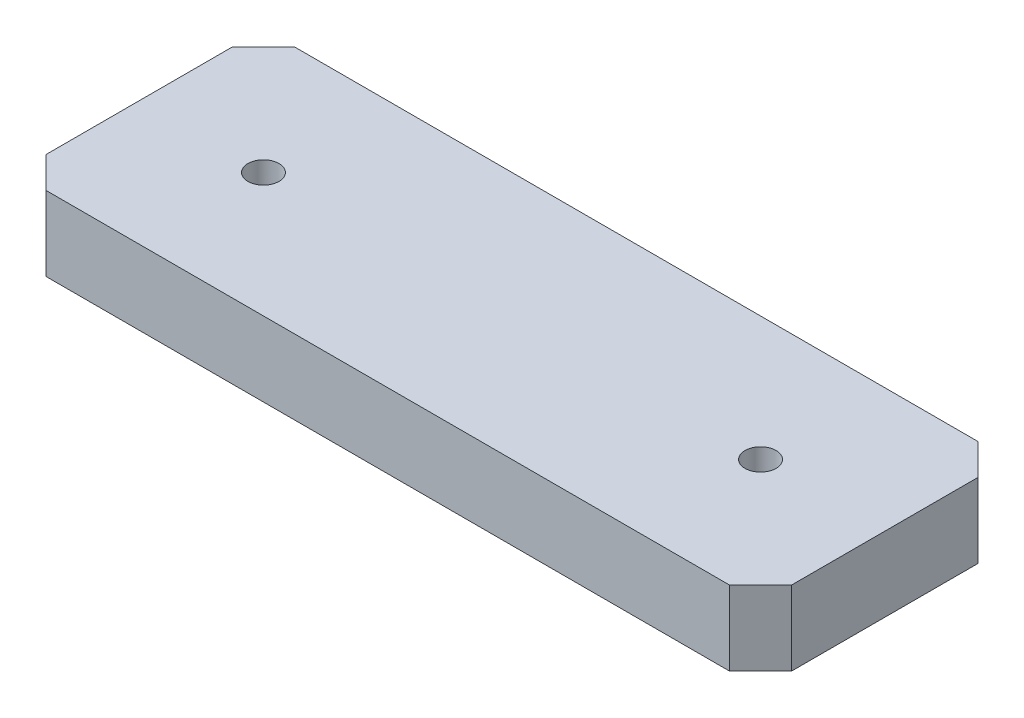
SolidWorks part; units mm, degrees
material "45#"
ref_plane "Front Plane" through (0, 0, 0) normal (0, 0, 1) x (1, 0, 0)
ref_plane "Top Plane" through (0, 0, 0) normal (0, 1, 0) x (1, 0, 0)
ref_plane "Right Plane" through (0, 0, 0) normal (1, 0, 0) x (0, 0, -1)
sketch "Sketch1" plane through (0, 0, 0) normal (0, 1, 0) x (1, 0, 0)
  line L0 (60, 20) -> (-60, -20) construction
  line L1 (-60, 20) -> (60, 20)
  line L2 (-60, 20) -> (-60, -20)
  line L3 (-60, -20) -> (60, -20)
  line L4 (60, 20) -> (60, -20)
  dimension "D1" = 120
  dimension "D2" = 40
extrude "Extrude1" add sketch "Sketch1" along normal mid plane 12
hole_wizard "M6 Tapped Hole1" positions "Sketch3" profile "Sketch2" tap size "M6" standard "ISO"
sketch "Sketch3" plane through (0, 6, 0) normal (0, 1, 0) x (-1, 0, 0)
  line L0 (-40, 0) -> (40, 0) construction
  line L2 (-60, 20) -> (-60, -20) construction
  point P0 (40, 0)
  point P1 (-40, 0)
  dimension "D1" = 20
sketch "Sketch2" plane through (-40, 6, 0) normal (1, 0, 0) x (0, 0, 1)
  line L0 (0, 0) -> (0, 16.5022)
  line L1 (0, 16.5022) -> (2.5, 15)
  line L2 (2.5, 15) -> (2.5, 0)
  line L5 (2.5, 0) -> (0, 0)
  line L10 (0, 16.5022) -> (-2.5, 15) construction
  line L11 (0, -6.35) -> (0, 107.95) construction
  dimension "螺孔鑽直徑" = 5
  dimension "螺孔鑽深度" = 15
  dimension "導頭角度" = 118
cosmetic thread "Cosmetic Thread1" parameters "D1"=12, "D2"=6
cosmetic thread "Cosmetic Thread2" parameters "D1"=12, "D2"=6
chamfer "Chamfer1" distance 5 angle 45 4 edges at (60, 0, 20) (-60, 0, 20) (-60, 0, -20) (60, 0, -20)
